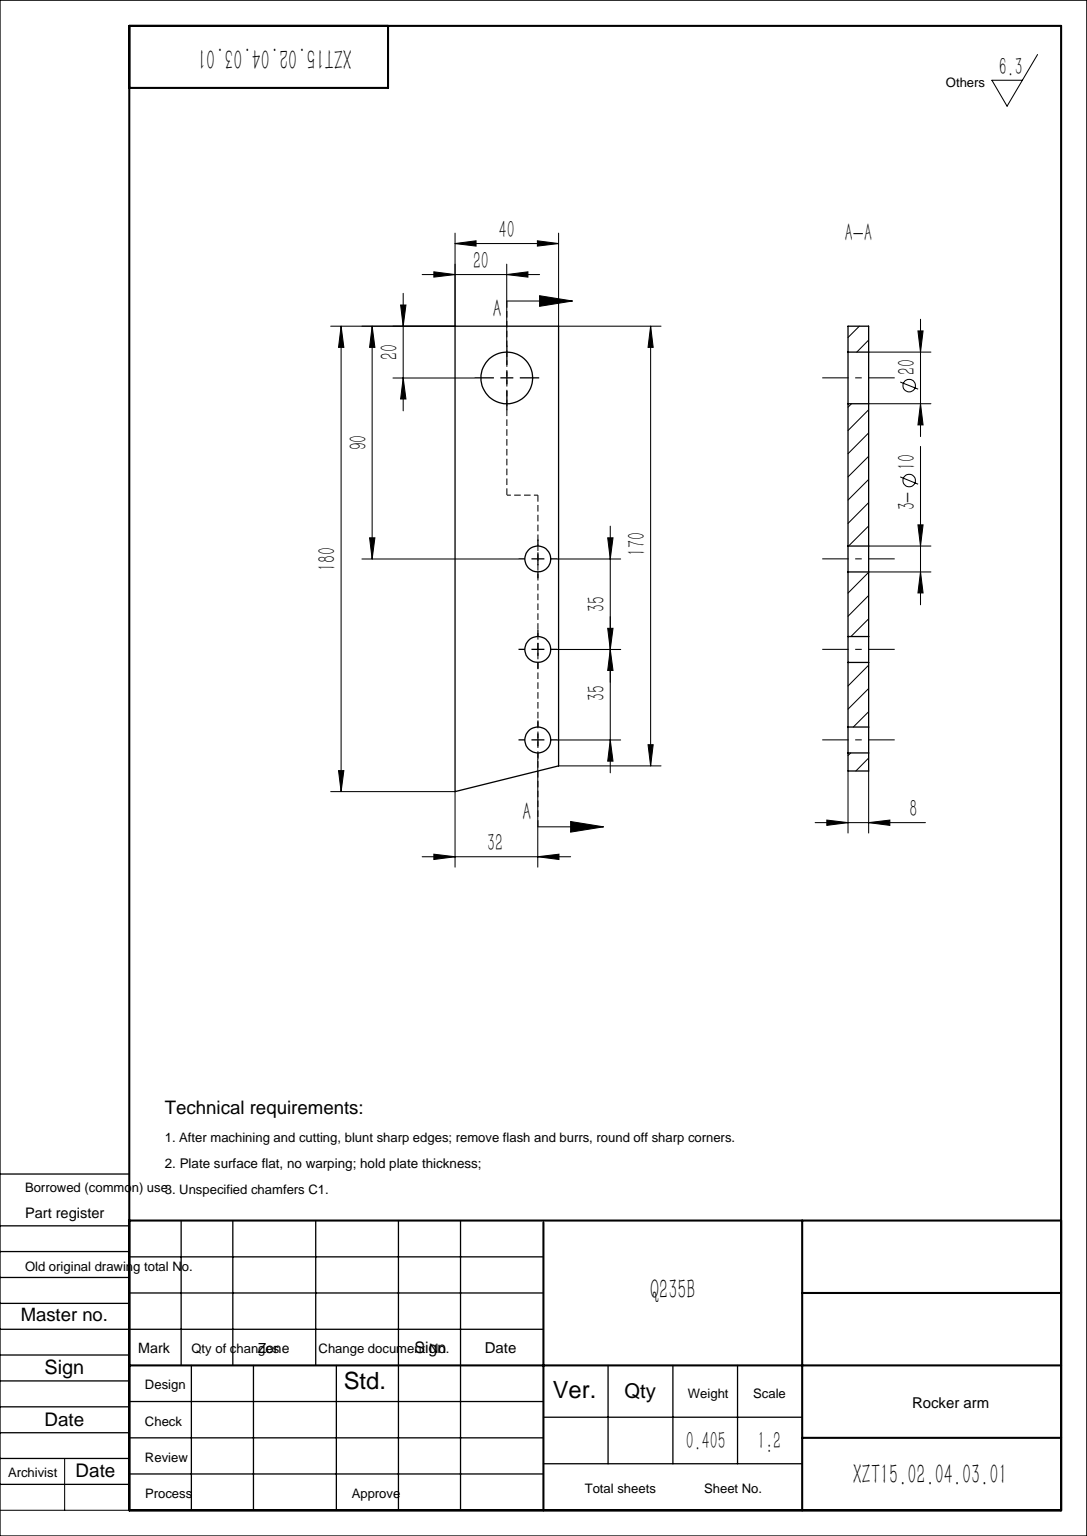
SolidWorks part; units mm, degrees
material "Q235B"
ref_plane "Front Plane" through (0, 0, 0) normal (0, 0, 1) x (1, 0, 0)
ref_plane "Top Plane" through (0, 0, 0) normal (0, 1, 0) x (1, 0, 0)
ref_plane "Right Plane" through (0, 0, 0) normal (1, 0, 0) x (0, 0, -1)
sketch "Sketch1" plane through (0, 0, 0) normal (0, 0, 1) x (1, 0, 0)
  line L0 (0, 0) -> (0, 180)
  line L1 (0, 180) -> (40, 180)
  line L2 (40, 180) -> (40, 10)
  line L3 (40, 10) -> (0, 0)
  line L4 (32, 90) -> (32, 55) construction
  circle A0 centre (20, 160) radius 10
  circle A1 centre (32, 90) radius 5
  circle A2 centre (32, 55) radius 5
  circle A3 centre (32, 20) radius 5
  dimension "D1" = 20
  dimension "D2" = 10
  dimension "D4" = 35
  dimension "D5" = 40
  dimension "D6" = 180
  dimension "D7" = 90
  dimension "D8" = 20
  dimension "D9" = 20
  dimension "D10" = 32
  dimension "D11" = 170
  dimension "D3" = 3
extrude "Boss-Extrude1" add sketch "Sketch1" along normal mid plane 8
